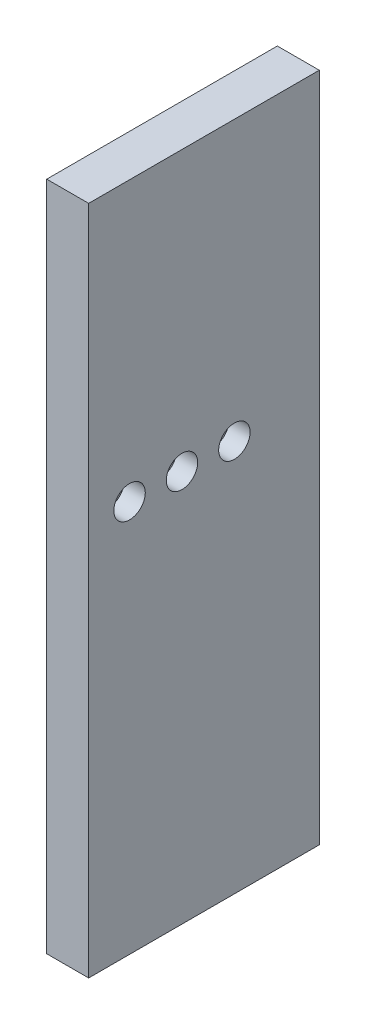
SolidWorks part; units mm, degrees
ref_plane "Front Plane" through (0, 0, 0) normal (0, 0, 1) x (1, 0, 0)
ref_plane "Top Plane" through (0, 0, 0) normal (0, 1, 0) x (1, 0, 0)
ref_plane "Right Plane" through (0, 0, 0) normal (1, 0, 0) x (0, 0, -1)
sketch "Sketch1" plane through (0, 0, 0) normal (0, 0, 1) x (1, 0, 0)
  line L0 (-120, 460) -> (255, 460) construction
  line L1 (100, 460) -> (120, 460)
  line L2 (100, 460) -> (100, 140)
  line L3 (100, 140) -> (120, 140)
  line L4 (120, 460) -> (120, 140)
  line L5 (-100, 460) -> (-100, 140) construction
  dimension "D1" = 20
  dimension "D2" = 320
  dimension "D3" = 200
extrude "Boss-Extrude1" add sketch "Sketch1" along normal blind 110
hole_wizard "CBORE for M10 Hex Head Bolt1" positions "Sketch2" profile "Sketch3" counterbore size "M10" standard "GB"
sketch "Sketch2" plane through (120, 0, 0) normal (1, 0, 0) x (0, 0, -1)
  point P0 (-90.49, 327)
  point P3 (-65.49, 327)
  point P6 (-40.49, 327)
sketch "Sketch3" plane through (120, 327, 90.49) normal (0, 1, 0) x (0, 0, -1)
  line L0 (0, 0) -> (0, 25.5547)
  line L1 (0, 25.5547) -> (5.5, 22.25)
  line L2 (5.5, 22.25) -> (5.5, 10)
  line L3 (5.5, 10) -> (7.5, 10)
  line L4 (7.5, 10) -> (7.5, 0)
  line L5 (7.5, 0) -> (0, 0)
  line L10 (0, 25.5547) -> (-5.5, 22.25) construction
  line L11 (0, -6.35) -> (0, 107.95) construction
  dimension "孔直径" = 11
  dimension "孔深度" = 22.25
  dimension "柱形沉头孔直径" = 15
  dimension "柱形沉头孔深度" = 10
  dimension "导头角度" = 118
